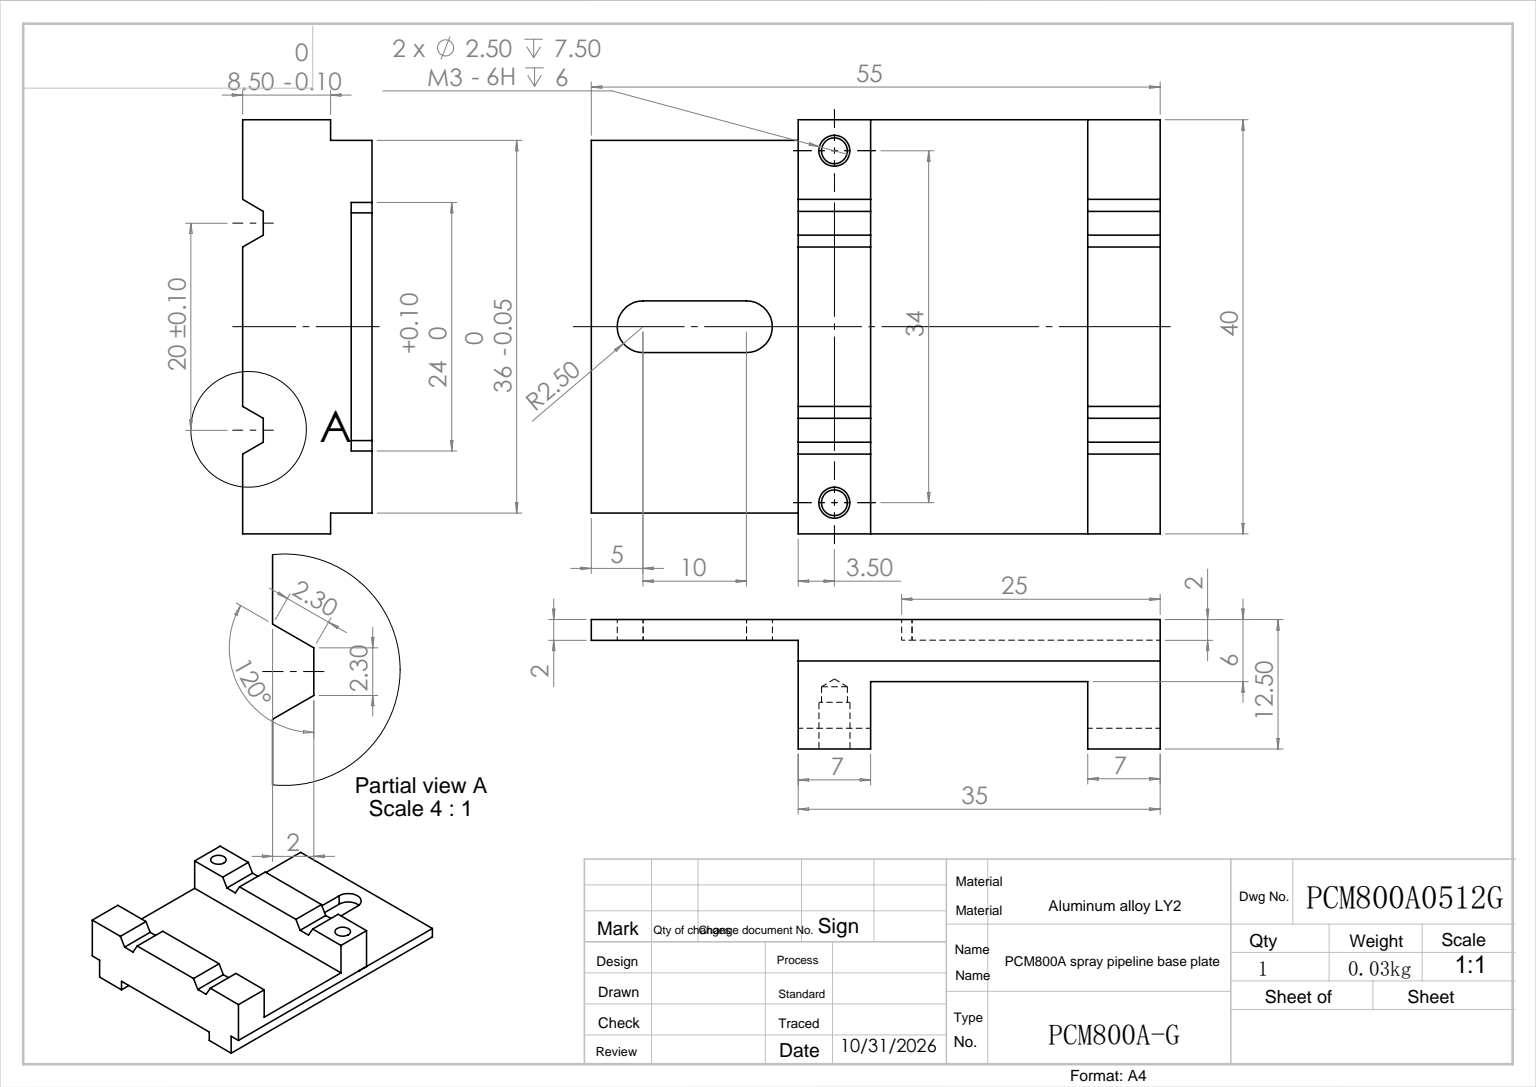
from build123d import *

# Parameters (mm, degrees)
SKETCH_1_W                   = 35
SKETCH_1_H                   = 4
EXTRUDE_1_DEPTH              = 40
SKETCH_2_W                   = 7
SKETCH_2_H                   = 40
EXTRUDE_2_DEPTH              = 12
HOLE_WIZARD_M3_1_D           = 2.5
HOLE_WIZARD_M3_1_DEPTH       = 7.5
HOLE_WIZARD_M3_1_CBORE_D     = 3
HOLE_WIZARD_M3_1_CBORE_DEPTH = 6
HOLE_WIZARD_M3_1_TIP         = 0.751075774
SKETCH_9_W                   = 7
SKETCH_9_H                   = 40
EXTRUDE_3_DEPTH              = 10
SKETCH_14_W                  = 40
SKETCH_14_H                  = 3.5
CUT_EXTRUDE_5_DEPTH          = 55.083269132
SKETCH_15_W                  = 2
SKETCH_15_H                  = 2
CUT_EXTRUDE_6_DEPTH          = 54.546708582
EXTRUDE_5_DEPTH              = 2
CUT_EXTRUDE_7_DEPTH          = 54.546708582
FILLET_1_R                   = 1
CUT_EXTRUDE_8_DEPTH          = 55.177947543


with BuildPart() as part:
    # 草图1 → 拉伸1 (new body)
    with BuildSketch(Plane.XY):
        with Locations((17.5, 2)):
            Rectangle(SKETCH_1_W, SKETCH_1_H)
    extrude(amount=EXTRUDE_1_DEPTH)

    # 草图2 → 拉伸2 (add)
    with BuildSketch(Plane(origin=(0, 4, 0), x_dir=(-1, 0, 0), z_dir=(0, 1, 0))):
        with Locations((-3.5, 20)):
            Rectangle(SKETCH_2_W, SKETCH_2_H)
    extrude(amount=-EXTRUDE_2_DEPTH)

    # M3 螺纹孔1
    with Locations(Plane.XZ.offset(8)):
        with Locations((3.5, 3), (3.5, 37)):
            CounterBoreHole(HOLE_WIZARD_M3_1_D / 2, HOLE_WIZARD_M3_1_CBORE_D / 2, HOLE_WIZARD_M3_1_CBORE_DEPTH, depth=HOLE_WIZARD_M3_1_DEPTH)
            with Locations((0, 0, -(HOLE_WIZARD_M3_1_DEPTH + HOLE_WIZARD_M3_1_TIP / 2))):  # 118° drill point
                Cone(0, HOLE_WIZARD_M3_1_D / 2, HOLE_WIZARD_M3_1_TIP, mode=Mode.SUBTRACT)

    # 草图9 → 拉伸3 (add)
    with BuildSketch(Plane.XZ):
        with Locations((31.5, 20)):
            Rectangle(SKETCH_9_W, SKETCH_9_H)
    extrude(amount=EXTRUDE_3_DEPTH)

    # 草图14 → 切除-拉伸5 (cut, through all)
    with BuildSketch(Plane(origin=(35, 0, 0), x_dir=(0, 0, -1), z_dir=(1, 0, 0))):
        with Locations((-20, -8.25)):
            Rectangle(SKETCH_14_W, SKETCH_14_H)
    extrude(amount=-CUT_EXTRUDE_5_DEPTH, mode=Mode.SUBTRACT)

    # 草图15 → 切除-拉伸6 (cut, through all)
    with BuildSketch(Plane.ZY):
        with Locations((1, 3)):
            Rectangle(SKETCH_15_W, SKETCH_15_H)
        with Locations((39, 3)):
            Rectangle(SKETCH_15_W, SKETCH_15_H)
    extrude(amount=-CUT_EXTRUDE_6_DEPTH, mode=Mode.SUBTRACT)

    # 草图17 → 拉伸5 (add)
    with BuildSketch(Plane(origin=(0, 4, 0), x_dir=(1, 0, 0), z_dir=(0, 1, 0))):
        Polygon((-20, -2), (35, -2), (35, -8), (10, -8), (10, -32), (35, -32), (35, -38), (-20, -38), align=None)
    extrude(amount=EXTRUDE_5_DEPTH)

    # 草图18 → 切除-拉伸7 (cut, through all)
    with BuildSketch(Plane.ZY):
        Polygon((31.15, -4.508141571), (28.85, -4.508141571), (27.7, -6.5), (28.85, -8.491858429), (31.15, -8.491858429), (32.3, -6.5), align=None)
    cut_extrude_7 = extrude(amount=-CUT_EXTRUDE_7_DEPTH, mode=Mode.SUBTRACT)

    # 镜向1: 切除-拉伸7 across plane
    add(cut_extrude_7.mirror(Plane(origin=(0, 0, 20), x_dir=(1, 0, 0), z_dir=(0, 0, -1))), mode=Mode.SUBTRACT)

    # 圆角1
    fillet_1_edges = [part.edges().sort_by_distance(p)[0] for p in [
        (10, 5, 32),
        (10, 5, 8),
    ]]
    fillet(fillet_1_edges, radius=FILLET_1_R)

    # 草图20 → 切除-拉伸8 (cut, through all)
    with BuildSketch(Plane.XZ.offset(-4)):
        with BuildLine():
            Line((-15, 22.5), (-5, 22.5))
            ThreePointArc((-5, 22.5), (-2.5, 20), (-5, 17.5))
            Line((-5, 17.5), (-15, 17.5))
            ThreePointArc((-15, 17.5), (-17.5, 20), (-15, 22.5))
        make_face()
    extrude(amount=-CUT_EXTRUDE_8_DEPTH, mode=Mode.SUBTRACT)


solid = part.part
